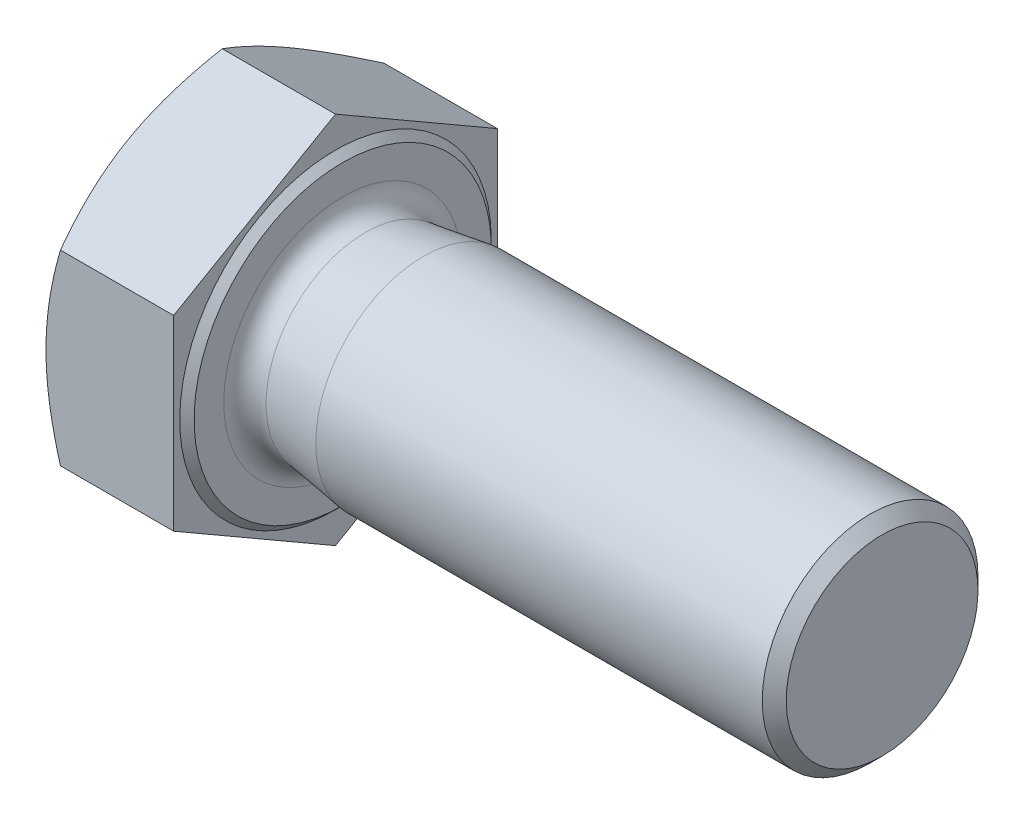
from build123d import *

# Parameters (mm, degrees)
EXTRUDE_1_DEPTH     = 15
SKETCH_4_R          = 39.55
SKETCH_4_R_2        = 18
CUT_EXTRUDE_1_DEPTH = 1.875
CUT_EXTRUDE_1_DRAFT = -60
CHAMFER_1_SIZE      = 1.333333333


with BuildPart() as part:
    # 草图3 → 凸台-拉伸1 (new body)
    with BuildSketch(Plane(origin=(0, 0, 0), x_dir=(0, 0, -1), z_dir=(1, 0, 0))):
        Polygon((18, 10.392304845), (0, 20.784609691), (-18, 10.392304845), (-18, -10.392304845), (0, -20.784609691), (18, -10.392304845), align=None)
    extrude(amount=EXTRUDE_1_DEPTH)


with BuildPart() as cut_extrude_1_tool:
    # 草图4 → 切除-拉伸1 (with draft: the straight prism first)
    with BuildSketch(Plane.ZY):
        Circle(SKETCH_4_R)
        Circle(SKETCH_4_R_2, mode=Mode.SUBTRACT)
    extrude(amount=-CUT_EXTRUDE_1_DEPTH)
    # 切除-拉伸1: the draft: its side faces are tilted about the plane it starts from
    cut_extrude_1_sides = [cut_extrude_1_tool.faces().sort_by_distance(p)[0] for p in [
        (0.9375, 0, -39.55),
        (0.9375, 0, -18),
    ]]
    draft(cut_extrude_1_sides, Plane.ZY, CUT_EXTRUDE_1_DRAFT)


with BuildPart() as part_1:
    add(part.part)

    # 切除-拉伸1: cut by cut_extrude_1_tool
    add(cut_extrude_1_tool.part, mode=Mode.SUBTRACT)

    # 草图6 → 旋转2 (revolve)
    with BuildSketch(Plane.XY, mode=Mode.PRIVATE) as revolve_2_sk:
        with BuildLine():
            Line((24, 12), (75, 12))
            Line((75, 12), (75, 0))
            Line((75, 0), (15, 0))
            Line((15, 0), (15, 13.22575))
            ThreePointArc((15, 13.22575), (15.76171636, 11.561015736), (17.519400155, 11.049059039))
            Line((17.519400155, 11.049059039), (24, 12))
        make_face()
    revolve(revolve_2_sk.sketch.rotate(Axis((15, 0, 0), (1, 0, 0)), 180), axis=Axis((15, 0, 0), (1, 0, 0)))

    # 倒角1
    chamfer_1_edges = [part_1.edges().sort_by_distance(p)[0] for p in [
        (75, 12, 0),
    ]]
    chamfer(chamfer_1_edges, length=CHAMFER_1_SIZE)

    # 草图8 → 切除-旋转2 (revolve, cut)
    with BuildSketch(Plane.XY, mode=Mode.PRIVATE) as cut_revolve_2_sk:
        Polygon((15, 16.525), (14.2, 17.325), (14.2, 39.55), (15, 39.55), align=None)
    revolve(cut_revolve_2_sk.sketch.rotate(Axis((0, 0, 0), (1, 0, 0)), 180), axis=Axis((0, 0, 0), (1, 0, 0)), mode=Mode.SUBTRACT)


solid = part_1.part
